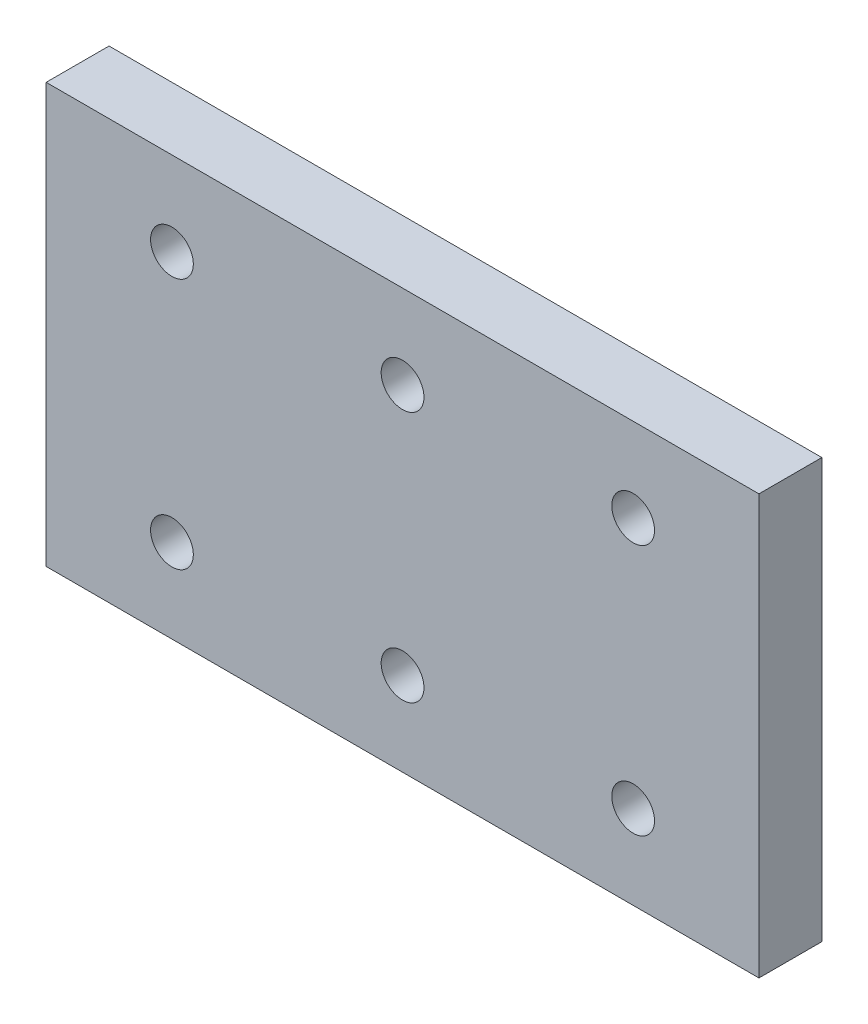
from build123d import *

# Parameters (mm, degrees)
SKETCH1_W              = 170
SKETCH1_H              = 100
BOSS_EXTRUDE1_DEPTH    = 15
M12_TAPPED_HOLE1_D     = 10.2
M12_TAPPED_HOLE1_DEPTH = 29.25
M12_TAPPED_HOLE1_TIP   = 3.064389157


with BuildPart() as part:
    # Sketch1 → Boss-Extrude1 (new body)
    with BuildSketch(Plane.XY):
        Rectangle(SKETCH1_W, SKETCH1_H)
    extrude(amount=BOSS_EXTRUDE1_DEPTH)

    # M12 Tapped Hole1
    with Locations(Plane.XY.offset(15)):
        with Locations((-55, 30), (0, 30), (55, 30), (55, -30), (0, -30), (-55, -30)):
            Hole(M12_TAPPED_HOLE1_D / 2, depth=M12_TAPPED_HOLE1_DEPTH)
            with Locations((0, 0, -(M12_TAPPED_HOLE1_DEPTH + M12_TAPPED_HOLE1_TIP / 2))):  # 118° drill point
                Cone(0, M12_TAPPED_HOLE1_D / 2, M12_TAPPED_HOLE1_TIP, mode=Mode.SUBTRACT)


solid = part.part
